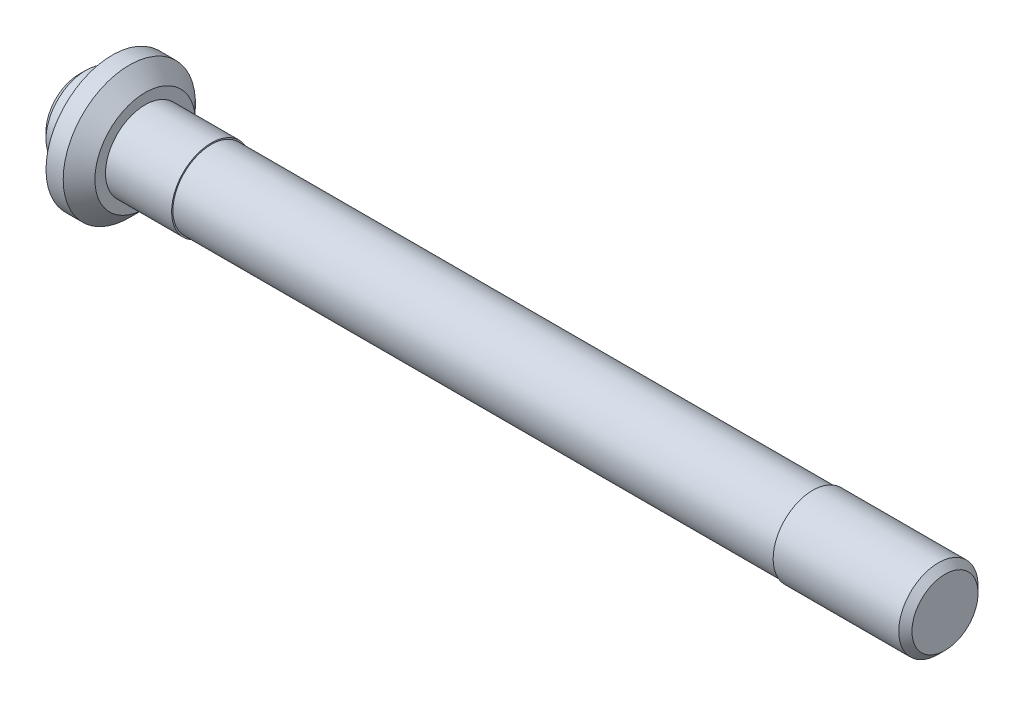
SolidWorks part; units mm, degrees
material "S45C"
ref_plane "Front Plane" through (0, 0, 0) normal (0, 0, 1) x (1, 0, 0)
ref_plane "Top Plane" through (0, 0, 0) normal (0, 1, 0) x (1, 0, 0)
ref_plane "Right Plane" through (0, 0, 0) normal (1, 0, 0) x (0, 0, -1)
sketch "Sketch1" plane through (0, 0, 0) normal (0, 0, 1) x (1, 0, 0)
  line L0 (0, 0) -> (61.1016, 0) construction
  line L1 (0, 0) -> (0, 3)
  line L2 (0, 3) -> (2.5, 3)
  line L3 (2.5, 3) -> (2.5, 5)
  line L4 (2.5, 5) -> (5, 5)
  line L5 (5, 5) -> (5, 3)
  line L6 (5, 3) -> (10, 3)
  line L7 (10, 3) -> (10, 2.9)
  line L8 (10, 2.9) -> (55.5, 2.9)
  line L9 (55.5, 2.9) -> (55.5, 3)
  line L10 (55.5, 3) -> (65.5, 3)
  line L11 (65.5, 3) -> (65.5, 0)
  line L12 (65.5, 0) -> (0, 0)
  dimension "D1" = 65.5
  dimension "D2" = 3
  dimension "D3" = 2.9
  dimension "D4" = 5
  dimension "D5" = 2.5
  dimension "D6" = 2.5
  dimension "D7" = 5
  dimension "D8" = 10
revolve "Revolve1" add sketch "Sketch1" angle 360 about L0
chamfer "Chamfer1" distance 1.2 angle 45 1 edges at (5, 0, 5)
hole_wizard "M3 Tapped Hole1" positions "Sketch3" profile "Sketch2" tap size "M3" standard "GB"
sketch "Sketch3" plane through (0, 0, 0) normal (-1, 0, 0) x (0, 0, 1)
  point P1 (0, 0)
sketch "Sketch2" plane through (0, 0, 0) normal (0, 1, 0) x (0, 0, 1)
  line L0 (0, 0) -> (0, 8.2511)
  line L1 (0, 8.2511) -> (1.25, 7.5)
  line L2 (1.25, 7.5) -> (1.25, 0)
  line L5 (1.25, 0) -> (0, 0)
  line L10 (0, 8.2511) -> (-1.25, 7.5) construction
  line L11 (0, -6.35) -> (0, 107.95) construction
  dimension "螺纹孔钻头直径" = 2.5
  dimension "螺纹孔钻头深度" = 7.5
  dimension "导头角度" = 118
cosmetic thread "Hole thread1" parameters "D1"=6, "D2"=3
chamfer "Chamfer2" distance 0.5 angle 45 2 edges at (0, 0, 3) (65.5, 0, 3)
